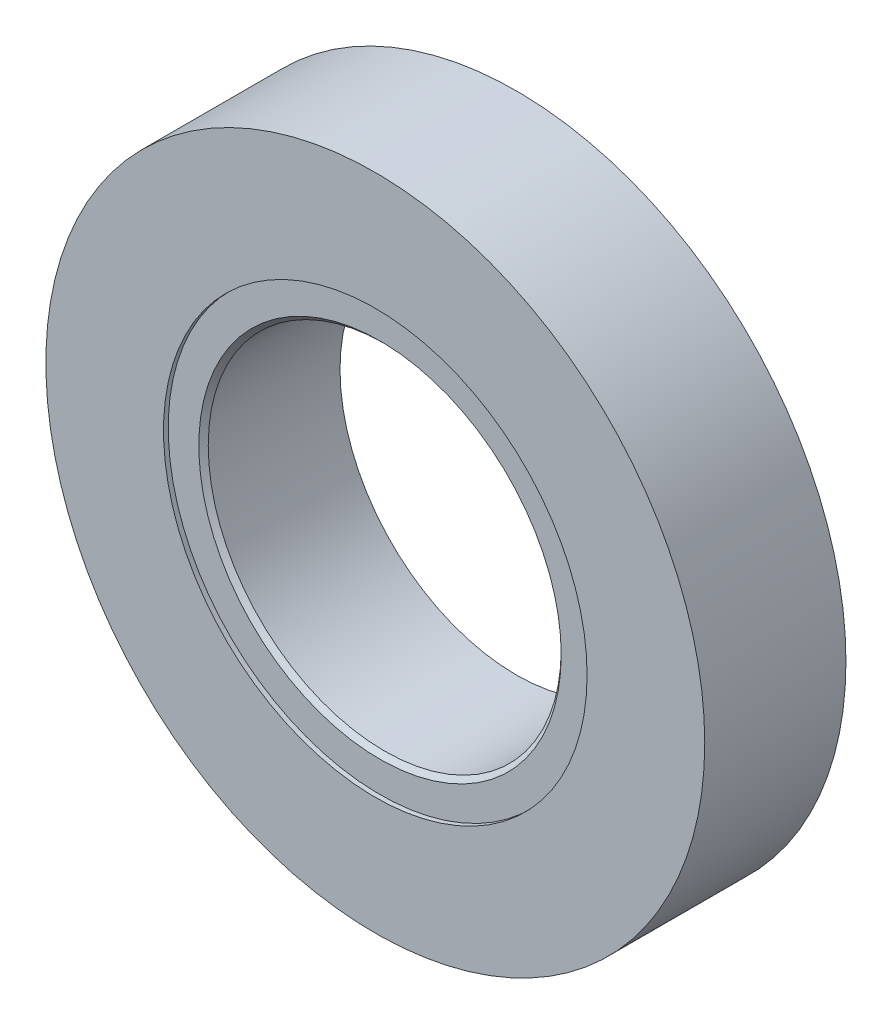
SolidWorks part; units mm, degrees
material "1023 碳钢板 (SS)"
ref_plane "前视基准面" through (0, 0, 0) normal (0, 0, 1) x (1, 0, 0)
ref_plane "上视基准面" through (0, 0, 0) normal (0, 1, 0) x (1, 0, 0)
ref_plane "右视基准面" through (0, 0, 0) normal (1, 0, 0) x (0, 0, -1)
sketch "草图1" plane through (0, 0, 0) normal (0, 0, 1) x (1, 0, 0)
  circle A0 centre (0, 0) radius 70
  circle A1 centre (0, 0) radius 37.5
  dimension "D1" = 140
  dimension "D2" = 75
extrude "凸台-拉伸1" add sketch "草图1" along normal blind 30 contours A0 | A1
sketch "草图2" plane through (0, 0, 30) normal (0, 0, 1) x (1, 0, 0)
  circle A0 centre (0, 0) radius 45
  dimension "D1" = 90
extrude "切除-拉伸1" cut sketch "草图2" against normal blind 1
chamfer "倒角1" distance 1 angle 45 1 edges at (37.5, 0, 29)
